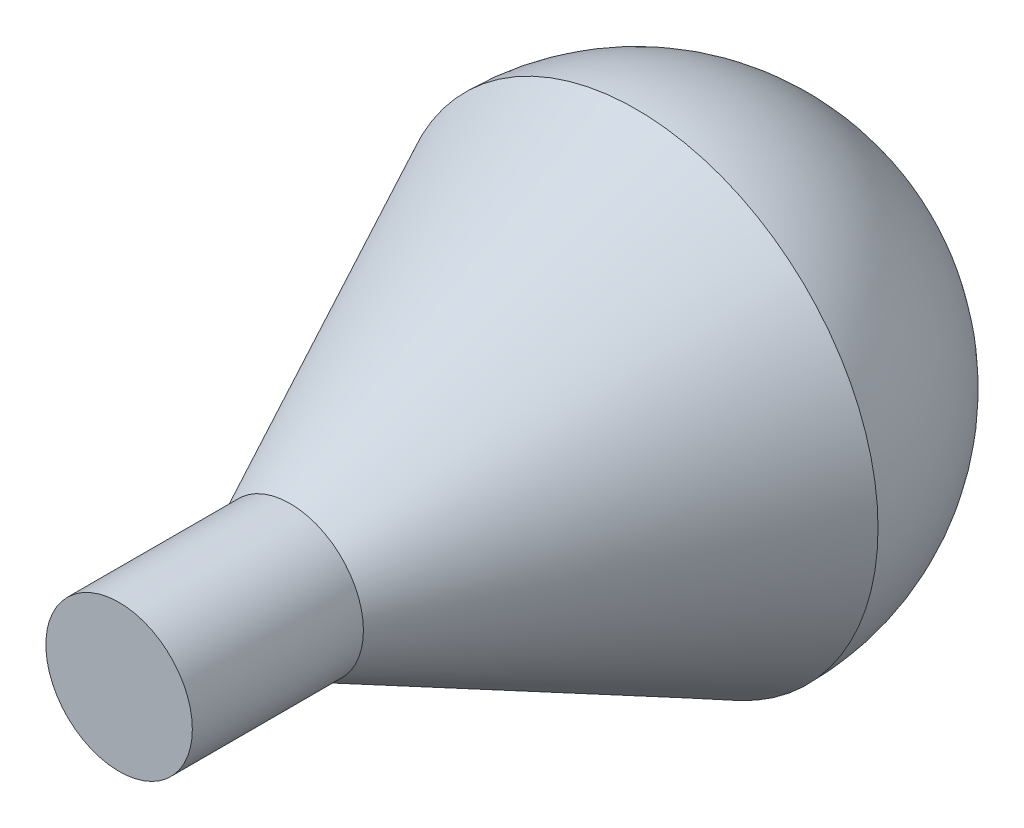
SolidWorks part; units mm, degrees
ref_plane "Front Plane" through (0, 0, 0) normal (0, 0, 1) x (1, 0, 0)
ref_plane "Top Plane" through (0, 0, 0) normal (0, 1, 0) x (1, 0, 0)
ref_plane "Right Plane" through (0, 0, 0) normal (1, 0, 0) x (0, 0, -1)
other "Configuration Table"
sketch "Sketch1" plane through (0, 0, 0) normal (0, 1, 0) x (1, 0, 0)
  line L0 (0, 0) -> (7.2399, 0)
  line L1 (7.2399, 0) -> (7.2399, 16.9122)
  line L2 (7.2399, 16.9122) -> (23.9104, 51.112)
  line L3 (0, 0) -> (0, 51.112)
  line L4 (0, 51.112) -> (0, 75.0224)
  arc A0 (23.9104, 51.112) -> (0, 75.0224) centre (0, 51.112) ccw
revolve "Revolve1" add sketch "Sketch1" angle 360 about L4
